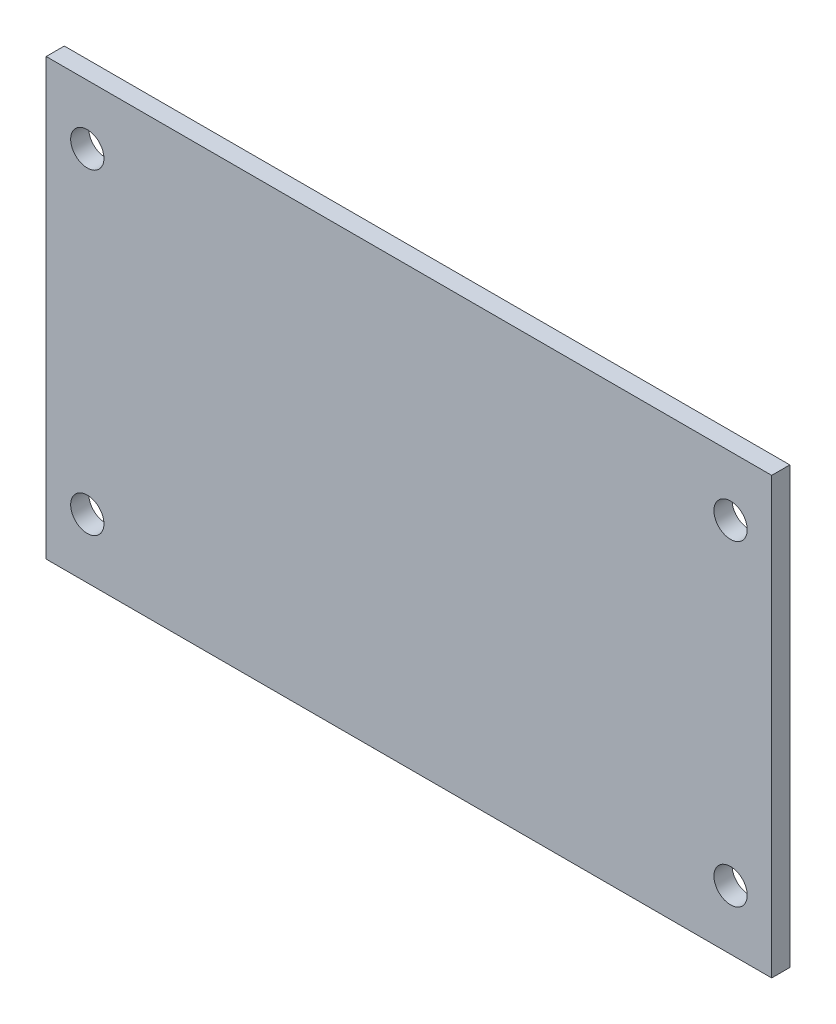
from build123d import *

# Parameters (mm, degrees)
SKETCH1_W            = 240
SKETCH1_H            = 144
BOSS_EXTRUDE1_DEPTH  = 6
SKETCH2_R            = 5.5
CUT_EXTRUDE1_DEPTH   = 6
LPATTERN1_COUNT      = 2
LPATTERN1_PITCH      = 212.8
LPATTERN1_COUNT_DIR2 = 2
LPATTERN1_PITCH_DIR2 = 104.7


with BuildPart() as part:
    # Sketch1 → Boss-Extrude1 (new body)
    with BuildSketch(Plane.XY):
        Rectangle(SKETCH1_W, SKETCH1_H)
    extrude(amount=BOSS_EXTRUDE1_DEPTH)

    # Sketch2 → Cut-Extrude1 (cut)
    with BuildSketch(Plane.XY.offset(6)):
        with Locations((-106.4, 52.35)):
            Circle(SKETCH2_R)
    cut_extrude1 = extrude(amount=-CUT_EXTRUDE1_DEPTH, mode=Mode.SUBTRACT)

    # LPattern1: Cut-Extrude1 2 × 2
    with Locations(*[(i * LPATTERN1_PITCH, -j * LPATTERN1_PITCH_DIR2, 0) for i in range(LPATTERN1_COUNT) for j in range(LPATTERN1_COUNT_DIR2) if (i, j) != (0, 0)]):
        add(cut_extrude1, mode=Mode.SUBTRACT)


solid = part.part
